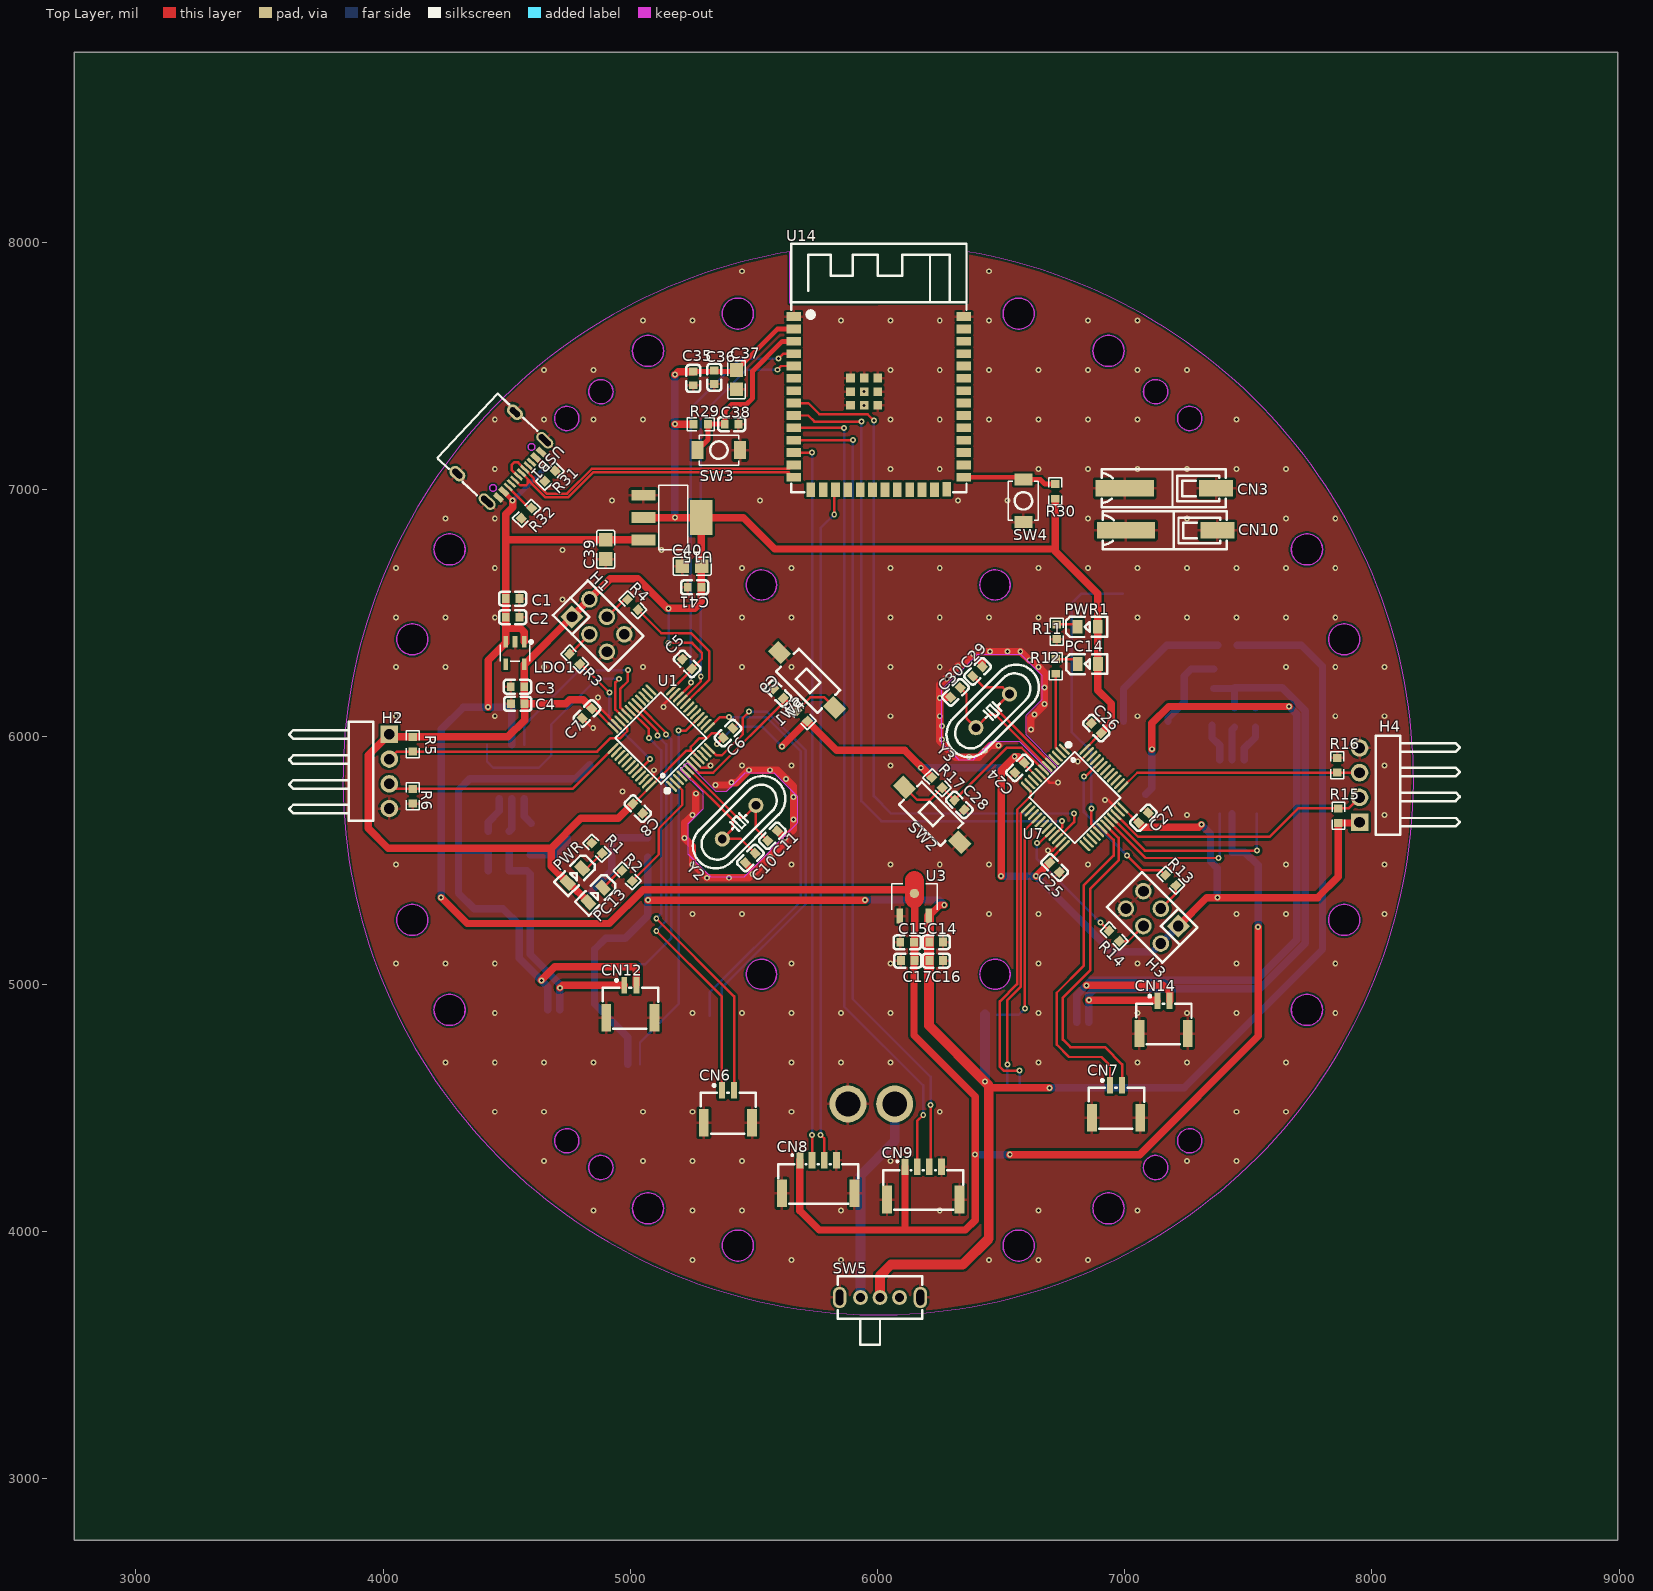
[diagram p0: Top Layer view]
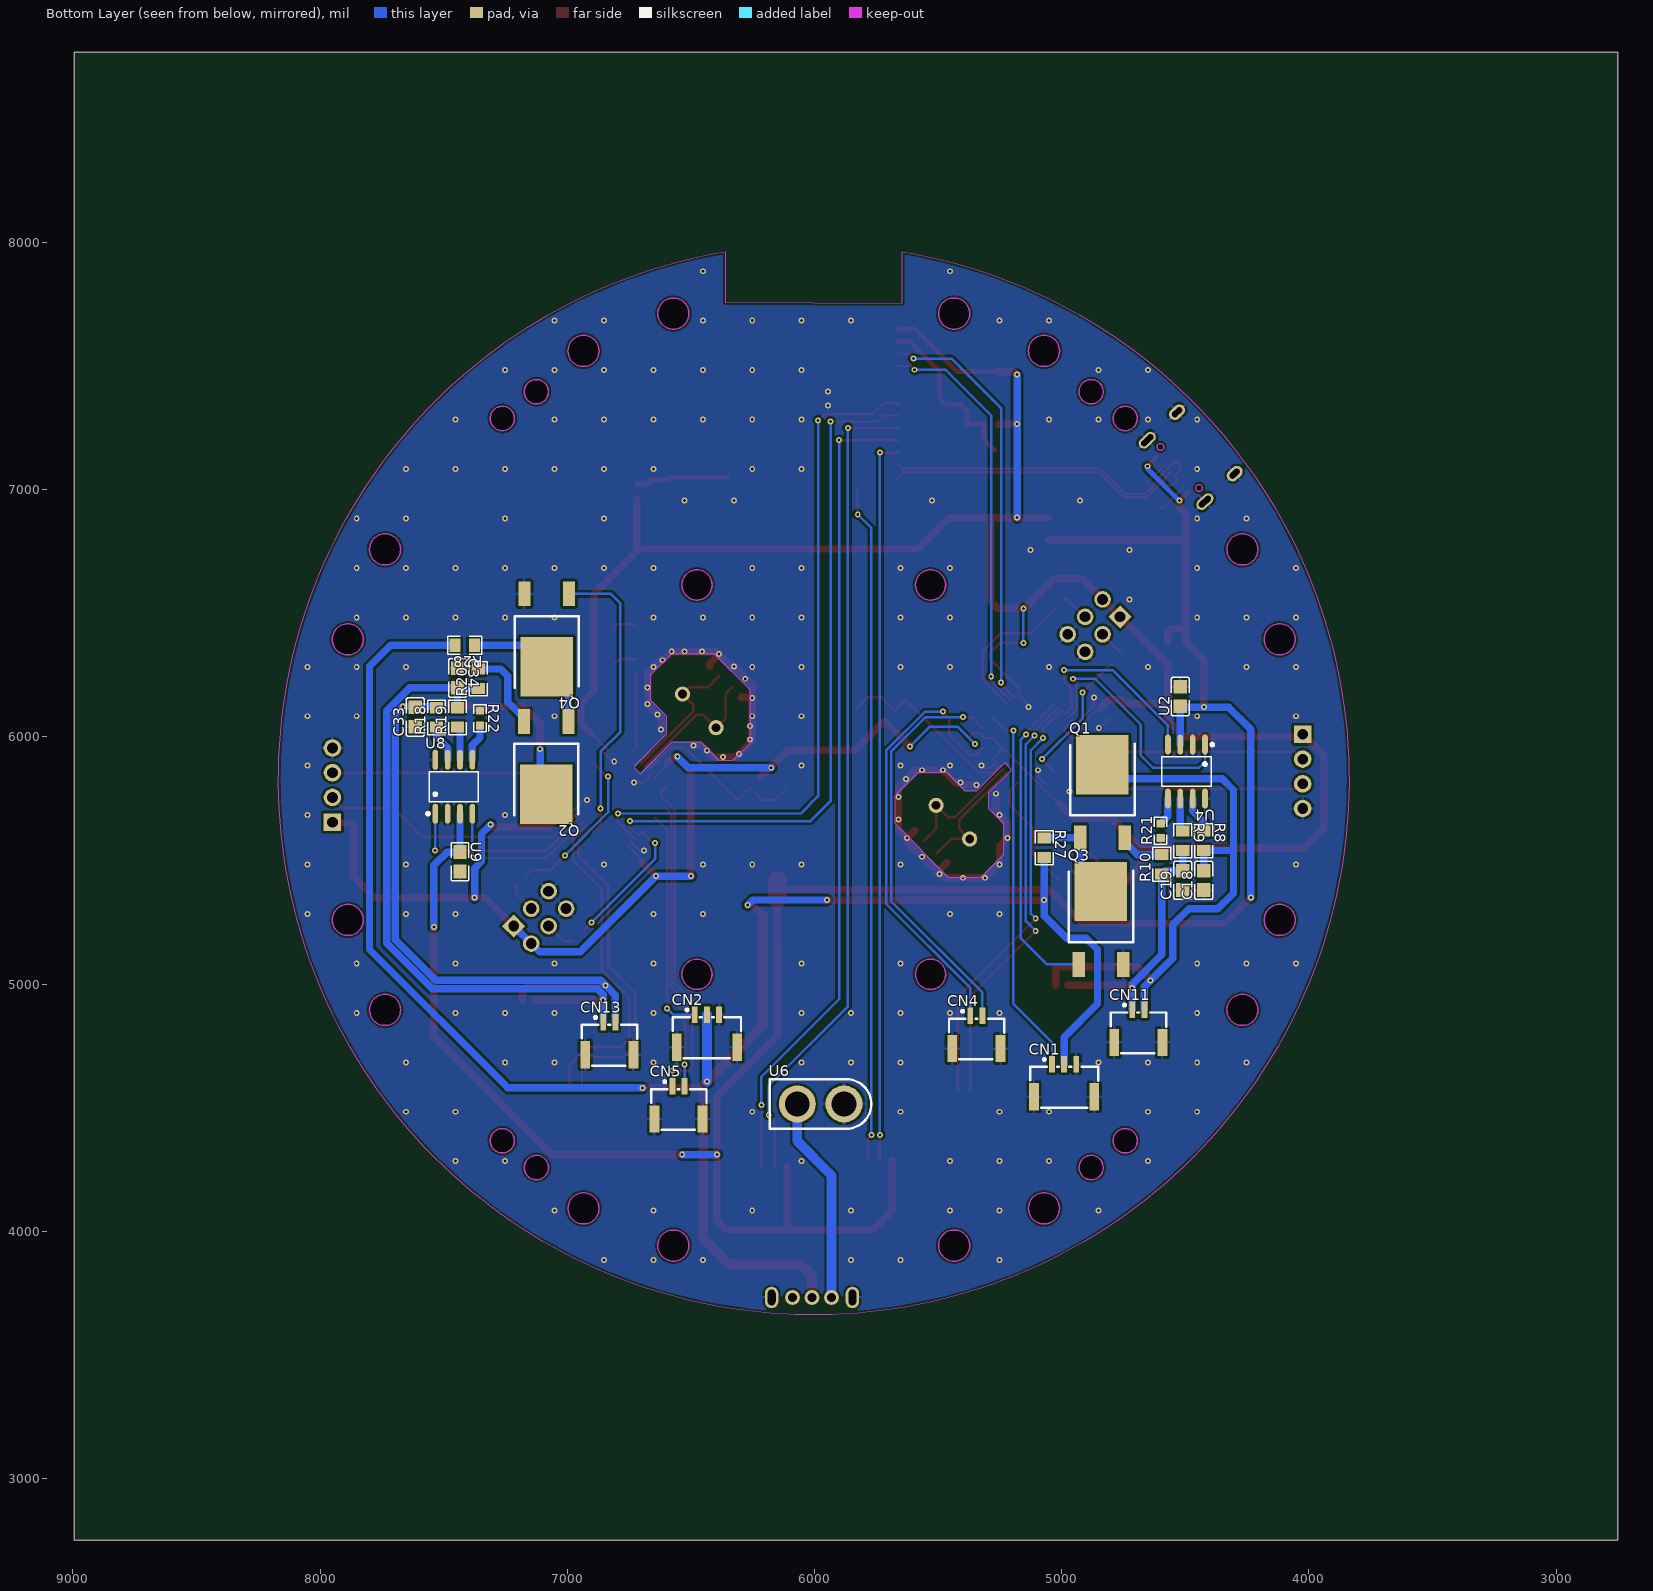
[diagram p1: Bottom Layer view, seen from below]
# Altium PCB MISC62500.pcbdoc (part 1 of 3)
Units mil, origin at the board's own origin, x right, y up, seen from the top; angles counter-clockwise.
Board outline 6245 x 6020 mil, 2 copper layers (Top Layer, Bottom Layer), stack 62.206 mil thick; 106 components, 73 nets, 432 pads, 293 vias.

## Layer stack, top to bottom
Top Solder Mask Layer: solder mask 0.394, Dk 3.3
Top Layer: signal copper 1.379
Dielectric1: surface 59.449, FR4, Dk 4.5
Bottom Layer: signal copper 1.378
Bottom Solder Mask Layer: solder mask 0.394, Dk 3.3

## Board outline
8995,2750 2750,2750 2750,8770 8995,8770
cut-out: 5591.53,5039.63 cw(c5530.51,5039.63) 5469.49,5039.63 cw(c5530.51,5039.63)
cut-out: 6536.44,6614.41 cw(c6475.41,6614.41) 6414.39,6614.41 cw(c6475.41,6614.41)
cut-out: 4792.31,4366.1 cw(c4743.1,4366.1) 4693.89,4366.1 cw(c4743.1,4366.1)
cut-out: 7174.2,4257.75 cw(c7124.98,4257.75) 7075.77,4257.75 cw(c7124.98,4257.75)
cut-out: 4930.15,7396.29 cw(c4880.94,7396.29) 4831.73,7396.29 cw(c4880.94,7396.29)
cut-out: 7312.03,7287.94 cw(c7262.82,7287.94) 7213.61,7287.94 cw(c7262.82,7287.94)
cut-out: 4181.09,6394.72 cw(c4118.1,6394.72) 4055.11,6394.72 cw(c4118.1,6394.72)
cut-out: 5498.26,3942.16 cw(c5435.26,3942.16) 5372.27,3942.16 cw(c5435.26,3942.16)
cut-out: 7950.82,5259.32 cw(c7887.83,5259.32) 7824.83,5259.32 cw(c7887.83,5259.32)
cut-out: 7174.24,7396.26 cw(c7125.03,7396.26) 7075.82,7396.26 cw(c7125.03,7396.26)
cut-out: 4331.76,6758.45 cw(c4268.77,6758.45) 4205.77,6758.45 cw(c4268.77,6758.45)
cut-out: 5134.53,4092.82 cw(c5071.53,4092.82) 5008.54,4092.82 cw(c5071.53,4092.82)
cut-out: 7800.15,4895.59 cw(c7737.16,4895.59) 7674.17,4895.59 cw(c7737.16,4895.59)
cut-out: 6633.65,7711.88 cw(c6570.66,7711.88) 6507.67,7711.88 cw(c6570.66,7711.88)
cut-out: 6997.38,7561.22 cw(c6934.39,7561.22) 6871.4,7561.22 cw(c6934.39,7561.22)
cut-out: 7950.83,6394.66 cw(c7887.84,6394.66) 7824.85,6394.66 cw(c7887.84,6394.66)
cut-out: 6633.6,3942.14 cw(c6570.6,3942.14) 6507.61,3942.14 cw(c6570.6,3942.14)
cut-out: 4181.07,5259.38 cw(c4118.08,5259.38) 4055.09,5259.38 cw(c4118.08,5259.38)
cut-out: 5498.31,7711.9 cw(c5435.32,7711.9) 5372.33,7711.9 cw(c5435.32,7711.9)
cut-out: 7800.18,6758.4 cw(c7737.18,6758.4) 7674.19,6758.4 cw(c7737.18,6758.4)
cut-out: 6997.33,4092.8 cw(c6934.34,4092.8) 6871.35,4092.8 cw(c6934.34,4092.8)
cut-out: 4331.73,4895.64 cw(c4268.74,4895.64) 4205.75,4895.64 cw(c4268.74,4895.64)
cut-out: 5134.58,7561.24 cw(c5071.58,7561.24) 5008.59,7561.24 cw(c5071.58,7561.24)
cut-out: 4792.35,7287.98 cw(c4743.14,7287.98) 4693.93,7287.98 cw(c4743.14,7287.98)
cut-out: 7311.99,4366.06 cw(c7262.78,4366.06) 7213.57,4366.06 cw(c7262.78,4366.06)
cut-out: 4930.11,4257.78 cw(c4880.89,4257.78) 4831.68,4257.78 cw(c4880.89,4257.78)
cut-out: 5591.56,6614.43 cw(c5530.53,6614.43) 5469.51,6614.43 cw(c5530.53,6614.43)
cut-out: 6536.41,5039.61 cw(c6475.39,5039.61) 6414.37,5039.61 cw(c6475.39,5039.61)

## Design rules (kind name [scope] priority, off if disabled: settings)
BoardOutlineClearance copperThickness2oz_1 [All] p2 off: genericclearance=8 ignorepadtopadclearanceinfootprint=FALSE except(0: Arc-SplitContinuation Track-SplitContinuation SMDPad-SplitContinuation THPad-SplitContinuation Via-SplitContinuation Fill-SplitContinuation Region-SplitContinuation Poly-SplitContinuation Text-SplitContinuation Hole-SplitContinuation; 6: Arc-CutoutEdge Track-CutoutEdge SMDPad-CutoutEdge THPad-CutoutEdge Via-CutoutEdge Text-CutoutEdge; 6.9: Hole-OutlineEdge Hole-CutoutEdge; 10: Poly-OutlineEdge Poly-CutoutEdge; 11.8: Arc-OutlineEdge Track-OutlineEdge SMDPad-OutlineEdge THPad-OutlineEdge Via-OutlineEdge Fill-OutlineEdge Region-OutlineEdge Text-OutlineEdge Fill-CutoutEdge Region-CutoutEdge)
BoardOutlineClearance Plane_innerPlane_1 [All] p4 off: genericclearance=4 ignorepadtopadclearanceinfootprint=FALSE except(0: Arc-SplitContinuation Track-SplitContinuation SMDPad-SplitContinuation THPad-SplitContinuation Via-SplitContinuation Fill-SplitContinuation Region-SplitContinuation Poly-SplitContinuation Text-SplitContinuation Hole-SplitContinuation; 6: Arc-CutoutEdge Track-CutoutEdge SMDPad-CutoutEdge THPad-CutoutEdge Via-CutoutEdge Text-CutoutEdge; 6.9: Hole-OutlineEdge Hole-CutoutEdge; 10: Poly-OutlineEdge Poly-CutoutEdge; 11.8: Arc-OutlineEdge Track-OutlineEdge SMDPad-OutlineEdge THPad-OutlineEdge Via-OutlineEdge Fill-OutlineEdge Region-OutlineEdge Text-OutlineEdge Fill-CutoutEdge Region-CutoutEdge)
BoardOutlineClearance Copper_copperRegion_1 [All] p6 off: genericclearance=4 ignorepadtopadclearanceinfootprint=FALSE except(0: Arc-SplitContinuation Track-SplitContinuation SMDPad-SplitContinuation THPad-SplitContinuation Via-SplitContinuation Fill-SplitContinuation Region-SplitContinuation Poly-SplitContinuation Text-SplitContinuation Hole-SplitContinuation; 6: Arc-CutoutEdge Track-CutoutEdge SMDPad-CutoutEdge THPad-CutoutEdge Via-CutoutEdge Text-CutoutEdge; 6.9: Hole-OutlineEdge Hole-CutoutEdge; 10: Poly-OutlineEdge Poly-CutoutEdge; 11.8: Arc-OutlineEdge Track-OutlineEdge SMDPad-OutlineEdge THPad-OutlineEdge Via-OutlineEdge Fill-OutlineEdge Region-OutlineEdge Text-OutlineEdge Fill-CutoutEdge Region-CutoutEdge)
BoardOutlineClearance copperThickness1oz_1 [All] p8: genericclearance=4 ignorepadtopadclearanceinfootprint=FALSE except(0: Arc-SplitContinuation Track-SplitContinuation SMDPad-SplitContinuation THPad-SplitContinuation Via-SplitContinuation Fill-SplitContinuation Region-SplitContinuation Poly-SplitContinuation Text-SplitContinuation Hole-SplitContinuation; 6: Arc-CutoutEdge Track-CutoutEdge SMDPad-CutoutEdge THPad-CutoutEdge Via-CutoutEdge Text-CutoutEdge; 6.9: Hole-OutlineEdge Hole-CutoutEdge; 10: Poly-OutlineEdge Poly-CutoutEdge; 11.8: Arc-OutlineEdge Track-OutlineEdge SMDPad-OutlineEdge THPad-OutlineEdge Via-OutlineEdge Fill-OutlineEdge Region-OutlineEdge Text-OutlineEdge Fill-CutoutEdge Region-CutoutEdge)
Clearance copperThickness2oz [All] p1 off: gap=8 ignorepadtopadclearanceinfootprint=FALSE except(6: SMDPad-Track SMDPad-SMDPad THPad-Track SMDPad-THPad THPad-THPad Track-Via SMDPad-Via THPad-Via Via-Via Fill-SMDPad Region-SMDPad Fill-THPad Region-THPad Fill-Via Region-Via Fill-Fill Fill-Region Region-Region Arc-Track Arc-SMDPad Arc-THPad Arc-Via Fill-Arc Region-Arc Arc-Arc Text-Track SMDPad-Text Text-THPad Text-Via Fill-Text Region-Text Arc-Text Text-Text; 6.9: Hole-Track Hole-SMDPad Hole-THPad Hole-Via Fill-Hole Region-Hole Hole-Arc Hole-Text; 10: Poly-Track Poly-SMDPad Poly-THPad Poly-Via Poly-Fill Poly-Region Poly-Poly Poly-Arc Poly-Text Poly-Hole; 11.8: Fill-Track Region-Track)
Clearance Plane_innerPlane [All] p3 off: gap=4 ignorepadtopadclearanceinfootprint=FALSE except(6: SMDPad-Track SMDPad-SMDPad THPad-Track SMDPad-THPad THPad-THPad Track-Via SMDPad-Via THPad-Via Via-Via Fill-SMDPad Region-SMDPad Fill-THPad Region-THPad Fill-Via Region-Via Fill-Fill Fill-Region Region-Region Arc-Track Arc-SMDPad Arc-THPad Arc-Via Fill-Arc Region-Arc Arc-Arc Text-Track SMDPad-Text Text-THPad Text-Via Fill-Text Region-Text Arc-Text Text-Text; 6.9: Hole-Track Hole-SMDPad Hole-THPad Hole-Via Fill-Hole Region-Hole Hole-Arc Hole-Text; 10: Poly-Track Poly-SMDPad Poly-THPad Poly-Via Poly-Fill Poly-Region Poly-Poly Poly-Arc Poly-Text Poly-Hole; 11.8: Fill-Track Region-Track)
Clearance Copper_copperRegion [All] p5 off: gap=4 ignorepadtopadclearanceinfootprint=FALSE except(6: SMDPad-Track SMDPad-SMDPad THPad-Track SMDPad-THPad THPad-THPad Track-Via SMDPad-Via THPad-Via Via-Via Fill-SMDPad Region-SMDPad Fill-THPad Region-THPad Fill-Via Region-Via Fill-Fill Fill-Region Region-Region Arc-Track Arc-SMDPad Arc-THPad Arc-Via Fill-Arc Region-Arc Arc-Arc Text-Track SMDPad-Text Text-THPad Text-Via Fill-Text Region-Text Arc-Text Text-Text; 6.9: Hole-Track Hole-SMDPad Hole-THPad Hole-Via Fill-Hole Region-Hole Hole-Arc Hole-Text; 10: Poly-Track Poly-SMDPad Poly-THPad Poly-Via Poly-Fill Poly-Region Poly-Poly Poly-Arc Poly-Text Poly-Hole; 11.8: Fill-Track Region-Track)
Clearance copperThickness1oz [All] p7: gap=4 ignorepadtopadclearanceinfootprint=FALSE except(6: SMDPad-Track SMDPad-SMDPad THPad-Track SMDPad-THPad THPad-THPad Track-Via SMDPad-Via THPad-Via Via-Via Fill-SMDPad Region-SMDPad Fill-THPad Region-THPad Fill-Via Region-Via Fill-Fill Fill-Region Region-Region Arc-Track Arc-SMDPad Arc-THPad Arc-Via Fill-Arc Region-Arc Arc-Arc Text-Track SMDPad-Text Text-THPad Text-Via Fill-Text Region-Text Arc-Text Text-Text; 6.9: Hole-Track Hole-SMDPad Hole-THPad Hole-Via Fill-Hole Region-Hole Hole-Arc Hole-Text; 10: Poly-Track Poly-SMDPad Poly-THPad Poly-Via Poly-Fill Poly-Region Poly-Poly Poly-Arc Poly-Text Poly-Hole; 11.8: Fill-Track Region-Track)
DiffPairsRouting differentialPair [All] p1: maxlimit=6 minlimit=6 mostfreqgap=6 toplayer_minwidth=5 toplayer_prefwidth=10 toplayer_maxwidth=100 toplayer_mingap=6 toplayer_prefgap=6 toplayer_maxgap=6 bottomlayer_minwidth=5 bottomlayer_prefwidth=10 bottomlayer_maxwidth=100 bottomlayer_mingap=6 bottomlayer_prefgap=6 bottomlayer_maxgap=6 maxuncoupledlength=10
HoleToHoleClearance otherClearance [All] p1: gap=11.8 allowstackedmicrovias=TRUE
Length netLength [All] p1: minlimit=0 maxlimit=0
PasteMaskExpansion pasteMaskExpansion [All] p1: expansion=0
PlaneConnect innerPlane [All] p1: planeconnectstyle=Relief reliefexpansion=20 reliefentries=4 reliefconductorwidth=10 reliefairgap=10
PolygonConnect copperRegion [All] p1: connectstyle=Relief reliefconductorwidth=10 reliefentries=4 polygonreliefangle="90 Angle" airgapwidth=10 via.connectstyle=Relief via.reliefconductorwidth=10 via.reliefentries=4 via.polygonreliefangle="90 Angle" via.airgapwidth=10
RoutingVias viaSize [All] p1: holewidth=12 width=24 viastyle="Through Hole" minholewidth=11.8 minwidth=19.7 maxholewidth=248 maxwidth=393.7
SolderMaskExpansion solderMaskExpansion [IsVia] p1: expansion=-1000 istentingtop=TRUE
SolderMaskExpansion solderMaskExpansion [All] p2: expansion=2 istentingtop=FALSE
Width copperThickness2oz_2 [All] p1 off: maxlimit=100 minlimit=8 preferedwidth=10
Width 5V [(InNet('+5V'))] p2: maxlimit=30 minlimit=15 preferedwidth=15
Width OUTPUT [(InNet('OUTPUT'))] p3: maxlimit=100 minlimit=30 preferedwidth=40
Width POWER [(InNet('POWER'))] p4: maxlimit=100 minlimit=40 preferedwidth=50
Width copperThickness1oz_2 [All] p5: maxlimit=30 minlimit=10 preferedwidth=10

## Components (designator, comment, footprint, x,y, rotation, side; value= is the part's Value field where it differs from the comment)
C1 "CAPCER0.1UF16VX5R0603,CAPCER0.1UF25VX5R0603,CAPCER0.1UF16VX7R0603" C0603 4523.68,6559.23 r180 top
C2 "1uF" C0603 4523.68,6484.23 r180 top
C3 "1uF" C0603 4543.75,6202.73 r0 top
C4 "CAPCER0.1UF16VX5R0603,CAPCER0.1UF25VX5R0603,CAPCER0.1UF16VX7R0603" C0603 4544.97,6133.68 r0 top
C5 "100nF" C0603 5230,6295 r315 top
C6 "100nF" C0603 5395,6015 r225 top
C7 "100nF" C0603 4825,6095 r45 top
C8 "100nF" C0603 5030,5710 r135 top
C9 "CAPCER0.1UF16VX5R0603,CAPCER0.1UF25VX5R0603,CAPCER0.1UF16VX7R0603" C0603 5598.98,6176.02 r315 top
C10 "18pF" C0603 5485,5510 r225 top
C11 "18pF" C0603 5575,5600 r45 top
C14 "100nF" C0603 6237.31,5169.82 r180 top
C15 "100nF" C0603 6119.9,5168.7 r180 top
C16 "10uF" C0603 6237.31,5094.82 r180 top
C17 "22uF" C0603 6122.31,5094.82 r180 top
C18 "30pF" C0805 4425.26,5419.55 r90 bottom
C19 "30pF" C0805 4510.26,5419.55 r90 bottom
C24 "100nF" C0603 6575,5875 r45 top
C25 "100nF" C0603 6716.52,5472.19 r135 top
C26 "100nF" C0603 6885,6035 r315 top
C27 "100nF" C0603 7075.5,5672.57 r225 top
C28 "CAPCER0.1UF16VX5R0603,CAPCER0.1UF25VX5R0603,CAPCER0.1UF16VX7R0603" C0603 6330.9,5724.96 r135 top
C29 "18pF" C0603 6405,6265 r45 top
C30 "18pF" C0603 6315,6180 r225 top
C33 "30pF" C0805 7615,6080 r90 bottom
C34 "30pF" C0805 7443.98,6238.37 r270 bottom
C35 "100nF" C0603 5255,7450 r90 top
C36 "100nF" C0603 5340,7455 r90 top
C37 "10uF" C0805 5430,7445 r90 top
C38 "100nF" C0603 5410,7265 r180 top
C39 "10uF" C0805 4900.52,6758.52 r90 top
C40 "22uF" C0805 5250,6690 r0 top
C41 "100nF" C0603 5260,6605 r180 top
CN1 "WAFER-GH1.25-3PLB" CONN-SMD_3P-P1.25_XUNPU_WAFER-GH1.25-3PLB 4990,4610 r180 bottom
CN2 "WAFER-GH1.25-3PLB" CONN-SMD_3P-P1.25_XUNPU_WAFER-GH1.25-3PLB 6435,4810.83 r180 bottom
CN3 "2060-451/998-404" CONN-SMD_L12.7-W3.9_2060-451-998-404 7185,7005 r0 top
CN4 "WAFER-GH1.25-2PLB" CONN-TH_2P-P1.25_XUNPU_WAFER-GH1.25-2PLB 5345,4805 r180 bottom
CN5 "WAFER-GH1.25-2PLB" CONN-TH_2P-P1.25_XUNPU_WAFER-GH1.25-2PLB 6550,4520 r180 bottom
CN6 "WAFER-GH1.25-2PLB" CONN-TH_2P-P1.25_XUNPU_WAFER-GH1.25-2PLB 5395,4505 r0 top
CN7 "WAFER-GH1.25-2PLB" CONN-TH_2P-P1.25_XUNPU_WAFER-GH1.25-2PLB 6965,4525 r0 top
CN8 "LQ-GH1.25-4PLT" CONN-SMD_LQ-GH1.25-4PLT 5760,4220 r0 top
CN9 "LQ-GH1.25-4PLT" CONN-SMD_LQ-GH1.25-4PLT 6185,4195 r0 top
CN10 "2060-451/998-404" CONN-SMD_L12.7-W3.9_2060-451-998-404 7190,6835 r0 top
CN11 "GH1.25-2P" CONN-TH_2P-P1.25_XUNPU_WAFER-GH1.25-2PLB 4690,4830 r180 bottom
CN12 "GH1.25-2P" CONN-TH_2P-P1.25_XUNPU_WAFER-GH1.25-2PLB 5000,4930 r0 top
CN13 "GH1.25-2P" CONN-TH_2P-P1.25_XUNPU_WAFER-GH1.25-2PLB 6830,4780 r180 bottom
CN14 "GH1.25-2P" CONN-TH_2P-P1.25_XUNPU_WAFER-GH1.25-2PLB 7156.97,4865.83 r0 top
H1 "PZ254V-12-6P" HDR-TH_6P-P2.54-V-M-R2-C3-S2.54 4870,6450 r315 top
H2 "2541WR-04P" HDR-TH_4P-P2.54-H-M-W10.4-N 4025,5860 r270 top
H3 "PZ254V-12-6P" HDR-TH_6P-P2.54-V-M-R2-C3-S2.54 7110.9,5269.96 r135 top
H4 "2541WR-04P" HDR-TH_4P-P2.54-H-M-W10.4-N 7950,5805 r90 top
LDO1 "ME6211C33M5G-N" SOT-23-5_L3.0-W1.7-P0.95-LS2.8-BL 4533.68,6339.23 r180 top
PC13 "NCD0805R1" LED0805-R-RD 4860,5360 r225 top
PC14 "NCD0805R1" LED0805-R-RD 6850.9,6294.96 r0 top
PWR "NCD0805R1" LED0805-R-RD 4775.81,5439.65 r225 top
PWR1 "NCD0805R1" LED0805-R-RD 6850,6445 r0 top
Q1 "STD12NF06LT4" TO-252-3_L6.5-W5.8-P4.58-BL 4835.26,5739.55 r180 bottom
Q2 "STD12NF06LT4" TO-252-3_L6.5-W5.8-P4.58-BL 7085,5915 r0 bottom
Q3 "STD12NF06LT4" TO-252-3_L6.5-W5.8-P4.58-BL 4841.07,5226.84 r180 bottom
Q4 "STD12NF06LT4" TO-252-3_L6.5-W5.8-P4.58-BL 7083.16,6431.07 r0 bottom
R1 "10kΩ" R0603 4865,5550 r135 top
R2 "10kΩ" R0603 4986.95,5438.05 r315 top
R3 "10kΩ" R0603 4775,6315 r135 top
R4 "10kΩ" R0603 5010,6535 r315 top
R5 "10kΩ" R0603 4120,5970 r90 top
R6 "10kΩ" R0603 4120.5,5759.88 r90 top
R7 "10kΩ" R0603 5695,6085 r315 top
R8 "0Ω" R0805 4425.26,5579.55 r270 bottom
R9 "0Ω" R0805 4510.26,5579.55 r270 bottom
R10 "120Ω" R0805 4595.26,5484.55 r90 bottom
R11 "10kΩ" R0603 6725,6425 r270 top
R12 "10kΩ" R0603 6720.9,6284.96 r270 top
R13 "10kΩ" R0603 7185.9,5419.96 r315 top
R14 "10kΩ" R0603 6957.24,5194.36 r135 top
R15 "10kΩ" R0603 7864.5,5681.24 r270 top
R16 "10kΩ" R0603 7860,5885 r270 top
R17 "10kΩ" R0603 6240.9,5814.96 r135 top
R18 "0Ω" R0805 7528.98,6078.37 r90 bottom
R19 "0Ω" R0805 7443.98,6078.37 r90 bottom
R20 "120Ω" R0805 7360,6235 r90 bottom
R21 "10kΩ" R0603 4600,5620 r90 bottom
R22 "10kΩ" R0603 7353.16,6076.07 r270 bottom
R27 "1kΩ" R0805 5071.07,5551.84 r270 bottom
R28 "1kΩ" R0805 7415,6370 r0 bottom
R29 "10kΩ" R0603 5285,7265 r0 top
R30 "10kΩ" R0603 6719.59,6992.67 r90 top
R31 "5.1kΩ" R0603 4675,7055 r225 top
R32 "5.1kΩ" R0603 4580,6905 r45 top
SW1 "TS-1101-C-W" SW-SMD_L6.0-W3.3-LS8.0 5715,6230 r135 top
SW2 "TS-1101-C-W" SW-SMD_L6.0-W3.3-LS8.0 6220.9,5684.96 r315 top
SW3 "TS-1088-AR02016" SW-SMD_L3.9-W3.0-P4.45 5357.96,7160 r180 top
SW4 "TS-1088-AR02016" SW-SMD_L3.9-W3.0-P4.45 6590,6955 r90 top
SW5 "SK12D07VG4" SW-TH_SK12D07VG4 6010,3732.22 r0 top
U1 "STM32F103C8T6" LQFP-48_L7.0-W7.0-P0.50-LS9.0-BL 5125,5995 r45 top
U2 "0.1uF/100V" C0805 4520.26,6163.29 r90 bottom
U3 "AMS1117-5.0" SOT-89-3_L4.5-W2.5-P1.50-LS4.2-BR 6149.06,5328.58 r270 top
U4 "TJA1050T/CM-YJLTY" SOIC-8_L4.9-W3.9-P1.27-LS6.0-BL 4495.26,5859.55 r0 bottom
U6 "XT30U-F" CONN-TH_XT30U-F 5975,4515 r180 bottom
U7 "STM32F103C8T6" LQFP-48_L7.0-W7.0-P0.50-LS9.0-BL 6797.3,5754.96 r225 top
U8 "TJA1050T/CM-YJLTY" SOIC-8_L4.9-W3.9-P1.27-LS6.0-BL 7458.98,5798.37 r180 bottom
U9 "0.1uF/100V" C0805 7433.98,5494.63 r270 bottom
U14 "2.4GHz" WIRELM-SMD_ESP32-S3-WROOM-1 6005,7350 r0 top
U15 "AMS1117-3.3" SOT-223-3_L6.5-W3.4-P2.30-LS7.0-BR 5169.97,6887.1 r180 top
USB1 "TYPE-C 16PIN 2MD(073)" USB-C-SMD_TYPE-C-16PIN-2MD-073 4485,7125 r226.8 top
Y2 "8M crystal" HC-49S_L11.5-W4.7-P4.88 5440,5655 r45 top
Y3 "8M crystal" HC-49S_L11.5-W4.7-P4.88 6465.9,6104.96 r225 top

## Footprints (in the part's own frame and the unit in brackets; to place one, negate y for a bottom-side part, rotate by r counter-clockwise, add the part's x,y. Pads: shape width x height; smd on the part's side, far side on the other; paste and mask are expansions set on the pad)
C0603 [mm]
  rect 0.8x0.9 smd: 1(-0.7,0) 2(0.7,0)
  silkscreen extent -1.41,-0.71 1.39,0.72
C0805 [mm]
  rect 1.41x1.35 smd paste-100 mask+0.051: 1(-1,0) 2(1,0)
  silkscreen extent -1.96,-0.9 1.96,0.9
CONN-SMD_3P-P1.25_XUNPU_WAFER-GH1.25-3PLB [mm]
  rect 0.6x1.7 smd: 1(-1.25,1.675) 2(0,1.675) 3(1.25,1.675)
  rect 1x2.8 smd: 4(3.1,-1.675) 5(-3.1,-1.675)
  silkscreen extent -3.5,-2.79 3.5,2.29
CONN-SMD_L12.7-W3.9_2060-451-998-404 [mm]
  rect 6x1.7 smd paste+0 mask+0.05: 1(-4.7,0)
  rect 3.5x1.7 smd paste+0 mask+0.05: 2(4.7,0)
  silkscreen extent -7.08,-1.95 5.67,1.95
CONN-SMD_LQ-GH1.25-4PLT [mm]
  rect 0.7x1.68 smd: 1(-1.875,1.692) 2(-0.625,1.692) 3(0.625,1.692) 4(1.875,1.692)
  rect 1x2.85 smd: 5(-3.725,-1.692) 6(3.725,-1.692)
  silkscreen extent -4.13,-2.76 4.12,2.33
CONN-TH_2P-P1.25_XUNPU_WAFER-GH1.25-2PLB [mm]
  rect 0.6x1.7 smd: 1(-0.625,1.675) 2(0.625,1.675)
  rect 1x2.8 smd: 3(2.475,-1.675) 4(-2.475,-1.675)
  silkscreen extent -2.81,-2.79 2.87,2.29
CONN-TH_XT30U-F [mm]
  round 3.8 hole 2.54: 1(2.4,0) 2(-2.4,0)
  silkscreen extent -5.21,-2.54 5.2,2.54
HC-49S_L11.5-W4.7-P4.88 [mm]
  round 1.56 hole 0.9: 1(-2.44,0) 2(2.44,0)
  silkscreen extent -5.75,-2.33 5.75,2.33
HDR-TH_4P-P2.54-H-M-W10.4-N [mm]
  rect 1.8x1.8 hole 1.1: 1(-3.81,0)
  round 1.8 hole 1.1: 2(-1.27,0) 3(1.27,0) 4(3.81,0)
  silkscreen extent -5.09,-10.27 5.07,-1.65
HDR-TH_6P-P2.54-V-M-R2-C3-S2.54 [mm]
  rect 1.7x1.7 hole 1.1: 1(-2.54,-1.27)
  round 1.7 hole 1.1: 2(-2.54,1.27) 3(0,-1.27) 4(0,1.27) 5(2.54,-1.27) 6(2.54,1.27)
  silkscreen extent -4.04,-2.54 4.04,2.54
LED0805-R-RD [mm]
  rect 1x1.4 smd: 1(1.05,0) 2(-1.05,0)
  silkscreen extent -2.22,-1.04 1.99,1.01
LQFP-48_L7.0-W7.0-P0.50-LS9.0-BL [mm]
  oval 0.27x1.5 smd paste+0 mask+0.05: 1(-2.75,-4.25) 2(-2.25,-4.25) 3(-1.75,-4.25) 4(-1.25,-4.25) 5(-0.75,-4.25) 6(-0.25,-4.25) 7(0.25,-4.25) 8(0.75,-4.25) 9(1.25,-4.25) 10(1.75,-4.25) 11(2.25,-4.25) 12(2.75,-4.25) 25(2.75,4.25) 26(2.25,4.25) 27(1.75,4.25) 28(1.25,4.25) 29(0.75,4.25) 30(0.25,4.25) 31(-0.25,4.25) 32(-0.75,4.25) 33(-1.25,4.25) 34(-1.75,4.25) 35(-2.25,4.25) 36(-2.75,4.25)
  oval 1.5x0.27 smd paste+0 mask+0.05: 13(4.25,-2.75) 14(4.25,-2.25) 15(4.25,-1.75) 16(4.25,-1.25) 17(4.25,-0.75) 18(4.25,-0.25) 19(4.25,0.25) 20(4.25,0.75) 21(4.25,1.25) 22(4.25,1.75) 23(4.25,2.25) 24(4.25,2.75) 37(-4.25,2.75) 38(-4.25,2.25) 39(-4.25,1.75) 40(-4.25,1.25) 41(-4.25,0.75) 42(-4.25,0.25) 43(-4.25,-0.25) 44(-4.25,-0.75) 45(-4.25,-1.25) 46(-4.25,-1.75) 47(-4.25,-2.25) 48(-4.25,-2.75)
  silkscreen extent -3.59,-4.46 3.3,3.34
R0603 [mil]
  rect 31.75x34.02 smd paste-3937.01 mask+2: 1(-29.66,0) 2(29.66,0)
  silkscreen extent -55,-26 55,26
R0805 [mm]
  rect 1.133x1.377 smd paste-100 mask+0.051: 1(-1,0) 2(1,0)
  silkscreen extent -1.76,-0.92 1.76,0.92
SOIC-8_L4.9-W3.9-P1.27-LS6.0-BL [mm]
  oval 0.588x2.045 smd: 1(-1.905,-2.772) 2(-0.635,-2.772) 3(0.635,-2.772) 4(1.905,-2.772) 5(1.905,2.772) 6(0.635,2.772) 7(-0.635,2.772) 8(-1.905,2.772)
  silkscreen extent -2.8,-2.92 2.53,1.52
SOT-23-5_L3.0-W1.7-P0.95-LS2.8-BL [mm]
  rect 0.49x1.157 smd: 1(-0.95,-1.154) 2(0,-1.154) 3(0.95,-1.154)
  rect 0.49x1.175 smd: 4(0.95,1.154) 5(-0.95,1.154)
  silkscreen extent -1.8,-1.29 1.53,0.85
SOT-89-3_L4.5-W2.5-P1.50-LS4.2-BR [mm]
  rect 1.575x0.672 smd: 1(1.356,-1.5) 3(1.356,1.5)
  round 0.95 smd: 2(-0.966,0)
  Top Layer region: -2.283,0.95 -0.429,0.95 -0.384,0.949 -0.34,0.946 -0.296,0.94 -0.252,0.933 -0.208,0.924 -0.165,0.912 -0.123,0.899 -0.081,0.884 -0.04,0.866 0,0.847 0.04,0.826 0.078,0.803 0.115,0.779 0.151,0.752 0.185,0.724 0.219,0.695 0.251,0.664 0.281,0.631 0.31,0.597 0.337,0.562 0.362,0.525 0.386,0.488 0.408,0.449 0.428,0.409 0.447,0.33 2.144,0.33 2.144,-0.33 0.447,-0.33 0.428,-0.409 0.408,-0.449 0.386,-0.488 0.362,-0.526 0.337,-0.562 0.31,-0.597 0.281,-0.631 0.251,-0.664 0.219,-0.695 0.185,-0.725 0.151,-0.753 0.115,-0.779 0.078,-0.804 0.04,-0.827 0,-0.848 -0.04,-0.867 -0.081,-0.884 -0.123,-0.899 -0.165,-0.913 -0.208,-0.924 -0.252,-0.934 -0.296,-0.941 -0.34,-0.946 -0.384,-0.949 -0.429,-0.95 -2.283,-0.95 -2.328,-0.949 -2.372,-0.946 -2.416,-0.941 -2.46,-0.934 -2.504,-0.924 -2.547,-0.913 -2.589,-0.899 -2.631,-0.884 -2.672,-0.867 -2.713,-0.848 -2.752,-0.827 -2.79,-0.804 -2.827,-0.779 -2.863,-0.753 -2.898,-0.725 -2.931,-0.695 -2.963,-0.664 -2.993,-0.631 -3.022,-0.597 -3.049,-0.562 -3.075,-0.526 -3.098,-0.488 -3.12,-0.449 -3.141,-0.409 -3.159,-0.369 -3.175,-0.327 -3.189,-0.285 -3.202,-0.242 -3.212,-0.199 -3.22,-0.155 -3.227,-0.111 -3.231,-0.067 -3.233,-0.022 -3.233,0.022 -3.231,0.067 -3.227,0.111 -3.22,0.155 -3.212,0.199 -3.202,0.242 -3.189,0.285 -3.175,0.327 -3.159,0.369 -3.141,0.409 -3.12,0.449 -3.098,0.488 -3.075,0.525 -3.049,0.562 -3.022,0.597 -2.993,0.631 -2.963,0.664 -2.931,0.695 -2.898,0.724 -2.863,0.752 -2.827,0.779 -2.79,0.803 -2.752,0.826 -2.713,0.847 -2.672,0.866 -2.631,0.884 -2.589,0.899 -2.547,0.912 -2.504,0.924 -2.46,0.933 -2.416,0.94 -2.372,0.946 -2.328,0.949
  silkscreen extent -1.95,-2.33 0.7,2.33
SOT-223-3_L6.5-W3.4-P2.30-LS7.0-BR [mm]
  rect 2.5x1.1 smd: 1(2.97,-2.3) 2(2.97,0) 3(2.97,2.3)
  rect 2.34x3.6 smd: 4(-2.97,0)
  silkscreen extent -1.57,-3.33 1.37,3.33
SW-SMD_L3.9-W3.0-P4.45 [mm]
  rect 1.23x1.86 smd: 1(-2.185,0) 2(2.185,0)
  silkscreen extent -2.03,-1.54 2.03,1.54
SW-SMD_L6.0-W3.3-LS8.0 [mm]
  rect 1.9x1.5 smd: 1(-4,0) 2(4,0)
  silkscreen extent -3.14,-1.67 2.86,1.63
SW-TH_SK12D07VG4 [mil]
  round 60 hole 36 paste+0 mask+1.97: 1(-78.74,0) 2(0,0) 3(78.74,0)
  oval 55.12x86.61 hole 31.5 slot 62.99 at 90 deg paste+0 mask+1.97: 4(163.38,0) 5(-163.39,0)
  silkscreen extent -171,-191 171,87
TO-252-3_L6.5-W5.8-P4.58-BL [mm]
  rect 1.27x2.54 smd: 1(-2.288,-3.747) 3(2.288,-3.745)
  rect 5.4x6.1 smd: 2(-0.002,3.747)
  silkscreen extent -3.31,-1.46 3.3,5.9
USB-C-SMD_TYPE-C-16PIN-2MD-073 [mm]
  oval 1.1x2 hole 0.6 slot 1.5 at 90.01 deg paste+0 mask+0.05: 13(-4.325,1.824) 14(4.325,1.826)
  oval 1.2x1.8 hole 0.6 slot 1.2 at 90.01 deg paste+0 mask+0.05: 13(-4.325,-2.376) 14(4.325,-2.374)
  rect 0.55x1.1 smd paste-100 mask+0.05: A1B12(-3.2,2.375) A4B9(-2.4,2.375) B1A12(3.2,2.375) B4A9(2.4,2.375)
  rect 0.3x1.1 smd paste-100 mask+0.05: A5(-1.25,2.375) A6(-0.25,2.375) A7(0.25,2.375) A8(1.25,2.375) B5(1.75,2.375) B6(0.75,2.375) B7(-0.75,2.375) B8(-1.75,2.375)
  Board Outline Layer circle w0.003: c-2.89,1.305 r0.35
  Board Outline Layer circle w0.003: c2.89,1.305 r0.35
  Board Outline Layer region: -3.13,1.56 -2.995,1.638 -2.84,1.651 -2.695,1.595 -2.588,1.481 -2.541,1.333 -2.563,1.179 -2.65,1.049 -2.65,1.049 -2.785,0.971 -2.94,0.958 -3.085,1.014 -3.192,1.128 -3.239,1.276 -3.217,1.43 -3.13,1.56
  Board Outline Layer region: -3.13,1.56 -3.067,1.607 -2.995,1.638 -2.918,1.653 -2.84,1.651 -2.764,1.631 -2.695,1.595 -2.635,1.544 -2.588,1.481 -2.556,1.41 -2.541,1.333 -2.544,1.254 -2.563,1.179 -2.6,1.109 -2.65,1.049 -2.713,1.002 -2.785,0.971 -2.862,0.956 -2.94,0.958 -3.016,0.978 -3.085,1.014 -3.145,1.065 -3.192,1.128 -3.224,1.199 -3.239,1.276 -3.236,1.355 -3.217,1.43 -3.18,1.5
  Board Outline Layer region: 2.65,1.56 2.785,1.639 2.94,1.652 3.085,1.596 3.192,1.482 3.239,1.334 3.217,1.179 3.13,1.05 3.13,1.05 2.995,0.971 2.84,0.959 2.695,1.015 2.588,1.128 2.541,1.277 2.563,1.431 2.65,1.56
  Board Outline Layer region: 2.65,1.56 2.713,1.607 2.785,1.639 2.862,1.654 2.94,1.652 3.016,1.632 3.085,1.596 3.145,1.545 3.192,1.482 3.224,1.41 3.239,1.334 3.236,1.255 3.217,1.179 3.18,1.11 3.13,1.05 3.067,1.003 2.995,0.971 2.918,0.956 2.84,0.959 2.764,0.979 2.695,1.015 2.635,1.066 2.588,1.128 2.556,1.2 2.541,1.277 2.544,1.355 2.563,1.431 2.6,1.501
  Multi-Layer board cut-out: -3.13,1.56 -2.995,1.638 -2.84,1.651 -2.695,1.595 -2.588,1.481 -2.541,1.333 -2.563,1.179 -2.65,1.049 -2.65,1.049 -2.785,0.971 -2.94,0.958 -3.085,1.014 -3.192,1.128 -3.239,1.276 -3.217,1.43 -3.13,1.56
  Multi-Layer board cut-out: 2.65,1.56 2.785,1.639 2.94,1.652 3.085,1.596 3.192,1.482 3.239,1.334 3.217,1.179 3.13,1.05 3.13,1.05 2.995,0.971 2.84,0.959 2.695,1.015 2.588,1.128 2.541,1.277 2.563,1.431 2.65,1.56
  silkscreen extent -4.5,-4.98 4.57,0.6
WIRELM-SMD_ESP32-S3-WROOM-1 [mm]
  rect 1.5x0.9 smd paste+0 mask+0.05: 1(-8.75,8.895) 2(-8.75,7.625) 3(-8.75,6.355) 4(-8.75,5.085) 5(-8.75,3.815) 6(-8.75,2.545) 7(-8.75,1.275) 8(-8.75,0.005) 9(-8.75,-1.265) 10(-8.75,-2.535) 11(-8.75,-3.805) 12(-8.75,-5.075) 13(-8.75,-6.345) 14(-8.75,-7.615) 27(8.75,-7.615) 28(8.75,-6.345) 29(8.75,-5.075) 30(8.75,-3.805) 31(8.75,-2.535) 32(8.75,-1.265) 33(8.75,0.005) 34(8.75,1.275) 35(8.75,2.545) 36(8.75,3.815) 37(8.75,5.085) 38(8.75,6.355) 39(8.75,7.625) 40(8.75,8.895)
  rect 0.9x1.5 smd paste+0 mask+0.05: 15(-6.985,-8.895) 16(-5.715,-8.895) 17(-4.445,-8.895) 18(-3.175,-8.895) 19(-1.905,-8.895) 20(-0.635,-8.895) 21(0.635,-8.895) 22(1.905,-8.895) 23(3.175,-8.895) 24(4.445,-8.895) 25(5.715,-8.895) 26(6.985,-8.865)
  rect 0.9x0.9 smd: 41(-2.9,-0.225) 41(-2.9,1.175) 41(-2.9,2.575) 41(-1.5,-0.225) 41(-1.5,1.175) 41(-1.5,2.575) 41(-0.1,-0.225) 41(-0.1,1.175) 41(-0.1,2.575)
  silkscreen extent -9,-9.14 9.02,16.39

## Via types
v1: diameter 24, hole 12, Top Layer to Bottom Layer, 293 vias